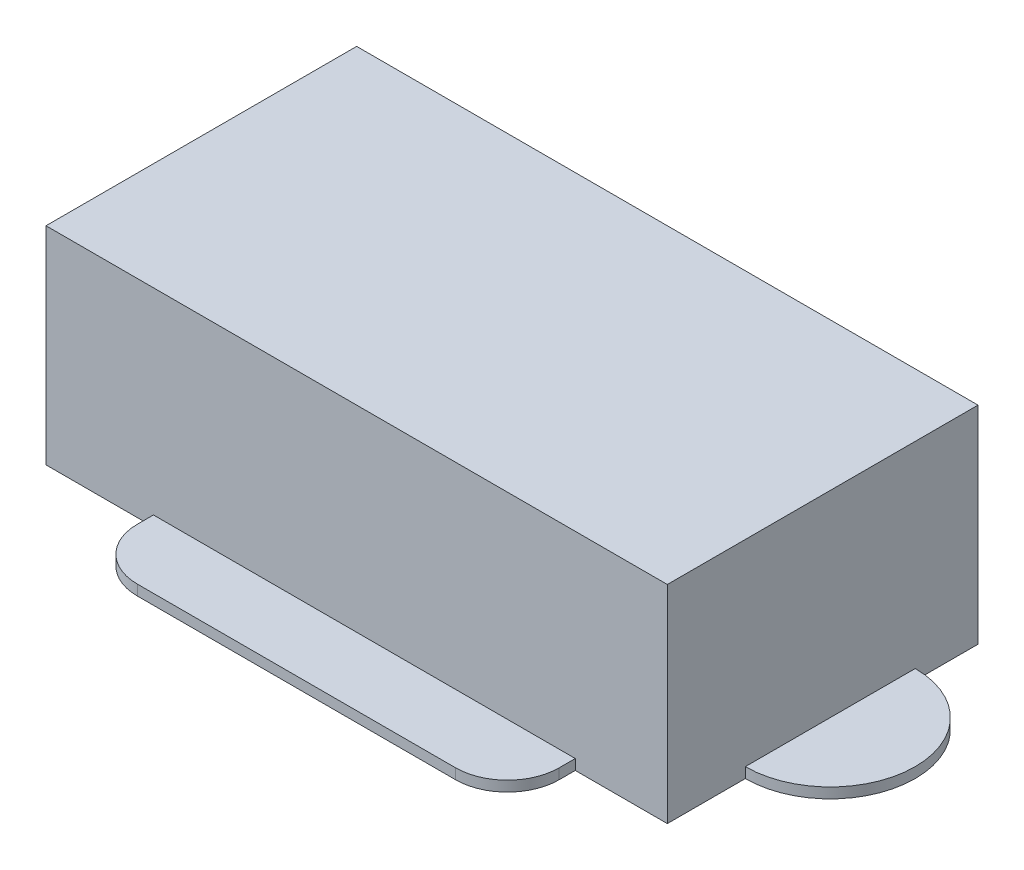
SolidWorks part; units mm, degrees
ref_plane "Front Plane" through (0, 0, 0) normal (0, 0, 1) x (1, 0, 0)
ref_plane "Top Plane" through (0, 0, 0) normal (0, 1, 0) x (1, 0, 0)
ref_plane "Right Plane" through (0, 0, 0) normal (1, 0, 0) x (0, 0, -1)
sketch "Sketch1" plane through (0, 0, 0) normal (0, 1, 0) x (1, 0, 0)
  line L1 (-30, 15) -> (30, 15)
  line L2 (-30, 15) -> (-30, -15)
  line L3 (-30, -15) -> (30, -15)
  line L4 (30, 15) -> (30, -15)
  line L5 (-30, 15) -> (30, -15) construction
  line L6 (-30, -15) -> (30, 15) construction
  point P0 (0, 0)
  dimension "D1" = 60
  dimension "D2" = 30
extrude "Boss-Extrude1" add sketch "Sketch1" along normal blind 20
sketch "Sketch2" plane through (0, 0, -15) normal (0, 0, -1) x (-1, 0, 0)
  line L1 (-18.753, 6.8134) -> (18.753, 6.8134)
  line L2 (-18.753, 6.8134) -> (-18.753, 13.0651)
  line L3 (-18.753, 13.0651) -> (18.753, 13.0651)
  line L4 (18.753, 6.8134) -> (18.753, 13.0651)
  line L5 (-18.753, 6.8134) -> (18.753, 13.0651) construction
  line L6 (-18.753, 13.0651) -> (18.753, 6.8134) construction
  point P0 (0, 9.9393)
extrude "Boss-Extrude2" add sketch "Sketch2" along normal blind 5
sketch "Sketch3" plane through (0, 0, 0) normal (0, -1, 0) x (1, 0, 0)
  line L0 (0, 0) -> (0, 32.7058) construction
  line L1 (-30, -15) -> (-30, 15) construction
  line L2 (-30, 7.473) -> (-30, -8.9398)
  line L3 (30, 7.473) -> (30, -8.9398)
  line L4 (-30, 15) -> (30, 15) construction
  line L5 (-19.6264, 15) -> (21.1099, 15)
  line L6 (-19.6264, 15) -> (-19.6264, 16.5561)
  line L7 (-14.6264, 21.5561) -> (16.1099, 21.5561)
  line L8 (21.1099, 15) -> (21.1099, 16.5561)
  arc A0 (-30, 7.473) -> (-30, -8.9398) centre (-30, -0.7334) ccw
  arc A1 (30, 7.473) -> (30, -8.9398) centre (30, -0.7334) cw
  arc A2 (21.1099, 16.5561) -> (16.1099, 21.5561) centre (16.1099, 16.5561) ccw
  arc A3 (-19.6264, 16.5561) -> (-14.6264, 21.5561) centre (-14.6264, 16.5561) cw
  dimension "D1" = 5
extrude "Boss-Extrude3" add sketch "Sketch3" against normal blind 1
